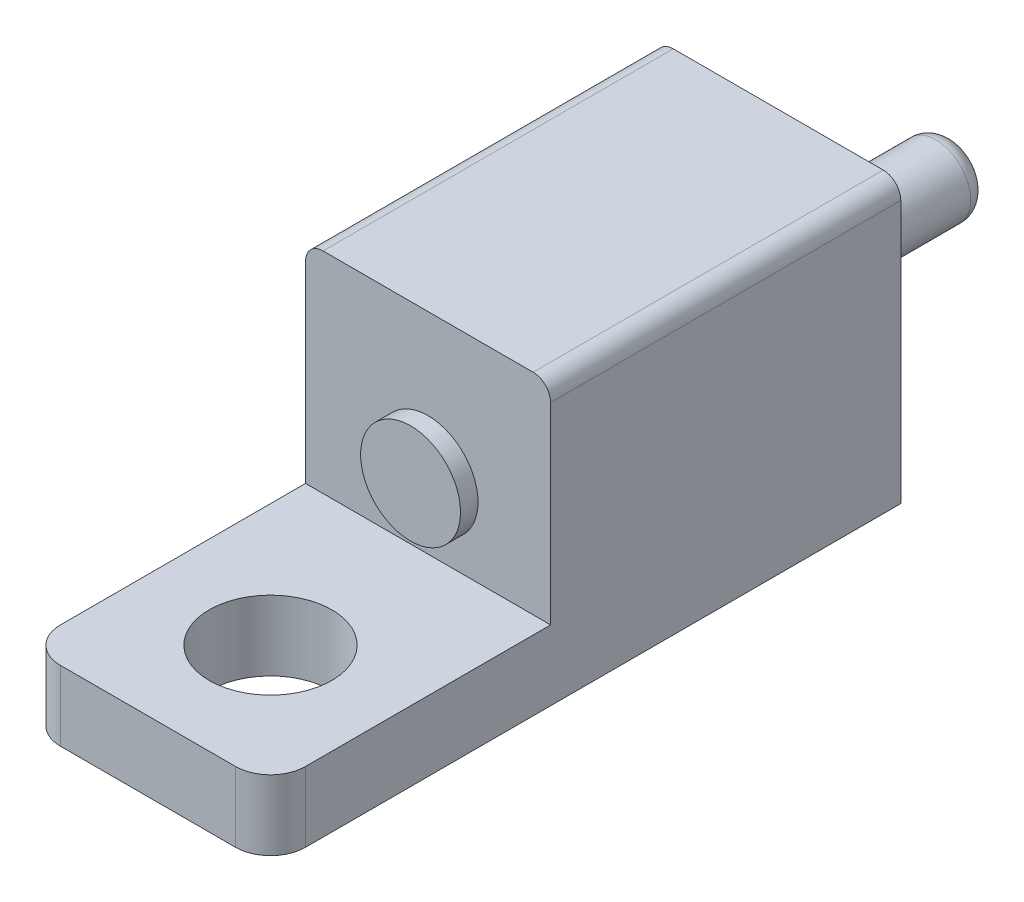
from build123d import *

# Parameters (mm, degrees)
SKETCH1_W           = 7
SKETCH1_H           = 8
BOSS_EXTRUDE1_DEPTH = 10
SKETCH2_W           = 7
SKETCH2_H           = 2
BOSS_EXTRUDE2_DEPTH = 8
SKETCH3_R           = 1
BOSS_EXTRUDE3_DEPTH = 5
FILLET1_R           = 0.5
SKETCH4_R           = 1.490192279
BOSS_EXTRUDE4_DEPTH = 1
SKETCH5_R           = 1.426715447
BOSS_EXTRUDE5_DEPTH = 0.5
FILLET3_R           = 0.5
FILLET4_R           = 1
SKETCH6_R           = 1.75
CUT_EXTRUDE1_DEPTH  = 20.293781382


with BuildPart() as part:
    # Sketch1 → Boss-Extrude1 (new body)
    with BuildSketch(Plane.XY):
        Rectangle(SKETCH1_W, SKETCH1_H)
    extrude(amount=BOSS_EXTRUDE1_DEPTH)

    # Sketch2 → Boss-Extrude2 (add)
    with BuildSketch(Plane.XY.offset(10)):
        with Locations((0, -3)):
            Rectangle(SKETCH2_W, SKETCH2_H)
    extrude(amount=BOSS_EXTRUDE2_DEPTH)

    # Sketch3 → Boss-Extrude3 (add)
    with BuildSketch(Plane(origin=(0, 0, 0), x_dir=(-1, 0, 0), z_dir=(0, 0, -1))):
        Circle(SKETCH3_R)
    extrude(amount=BOSS_EXTRUDE3_DEPTH)

    # Fillet1
    fillet1_edges = [part.edges().sort_by_distance(p)[0] for p in [
        (1, 0, -5),
    ]]
    fillet(fillet1_edges, radius=FILLET1_R)

    # Sketch4 → Boss-Extrude4 (add)
    with BuildSketch(Plane(origin=(0, 0, 0), x_dir=(-1, 0, 0), z_dir=(0, 0, -1))):
        with Locations(Location((0, 0, 0), (0, 0, 180))):
            Circle(SKETCH4_R)
    extrude(amount=BOSS_EXTRUDE4_DEPTH)

    # Sketch5 → Boss-Extrude5 (add)
    with BuildSketch(Plane.XY.offset(10)):
        Circle(SKETCH5_R)
    extrude(amount=BOSS_EXTRUDE5_DEPTH)

    # Fillet3
    fillet3_edges = [part.edges().sort_by_distance(p)[0] for p in [
        (-3.5, 4, 5),
        (3.5, 4, 5),
    ]]
    fillet(fillet3_edges, radius=FILLET3_R)

    # Fillet4
    fillet4_edges = [part.edges().sort_by_distance(p)[0] for p in [
        (3.5, -3, 18),
        (-3.5, -3, 18),
    ]]
    fillet(fillet4_edges, radius=FILLET4_R)

    # Sketch6 → Cut-Extrude1 (cut, through all)
    with BuildSketch(Plane(origin=(0, -2, 0), x_dir=(1, 0, 0), z_dir=(0, 1, 0))):
        with Locations(Location((0, -14.5, 0), (0, 0, 270))):
            Circle(SKETCH6_R)
    extrude(amount=-CUT_EXTRUDE1_DEPTH, mode=Mode.SUBTRACT)


solid = part.part
